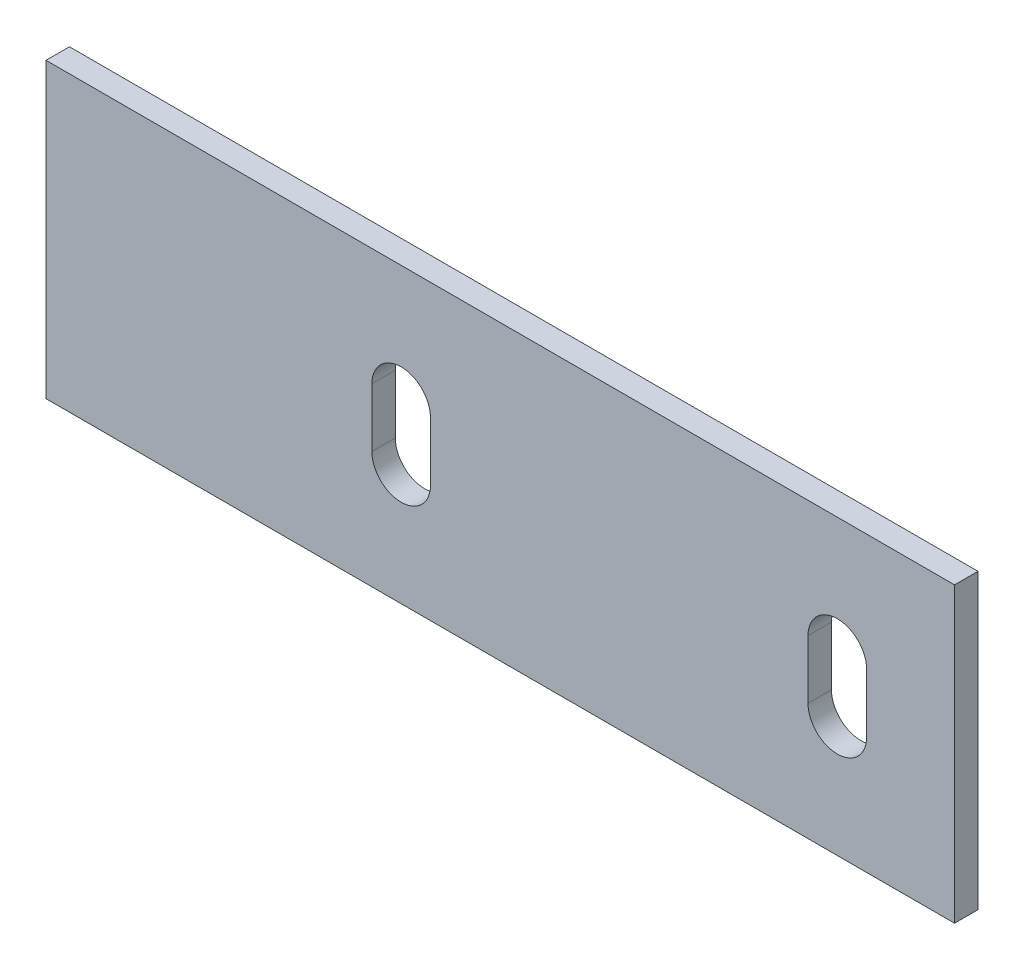
SolidWorks part; units mm, degrees
material "Q235B"
ref_plane "Front Plane" through (0, 0, 0) normal (0, 0, 1) x (1, 0, 0)
ref_plane "Top Plane" through (0, 0, 0) normal (0, 1, 0) x (1, 0, 0)
ref_plane "Right Plane" through (0, 0, 0) normal (1, 0, 0) x (0, 0, -1)
sketch "Sketch1" plane through (0, 0, 0) normal (0, 0, 1) x (1, 0, 0)
  line L0 (14040.3315, 4658.1603) -> (14040.3315, 4408.1603)
  line L1 (13265.2331, 4658.1603) -> (14040.3315, 4658.1603)
  line L2 (13265.2331, 4408.1603) -> (14040.3315, 4408.1603)
  line L3 (13265.2331, 4658.1603) -> (13265.2331, 4408.1603)
  line L4 (13543.2331, 4558.1603) -> (13543.2331, 4508.1603)
  line L5 (13593.2331, 4558.1597) -> (13593.2331, 4508.1605)
  line L6 (13915.3315, 4558.1603) -> (13915.3315, 4508.1603)
  line L7 (13965.3315, 4558.1597) -> (13965.3315, 4508.1605)
  arc A0 (13593.2331, 4558.1597) -> (13543.2331, 4558.1603) centre (13568.2331, 4558.16) ccw
  arc A1 (13543.2331, 4508.1603) -> (13593.2331, 4508.1605) centre (13568.2331, 4508.1603) ccw
  arc A2 (13965.3315, 4558.1597) -> (13915.3315, 4558.1603) centre (13940.3315, 4558.16) ccw
  arc A3 (13915.3315, 4508.1603) -> (13965.3315, 4508.1605) centre (13940.3315, 4508.1603) ccw
  dimension "D1" = 250
extrude "Boss-Extrude1" add sketch "Sketch1" along normal blind 20
